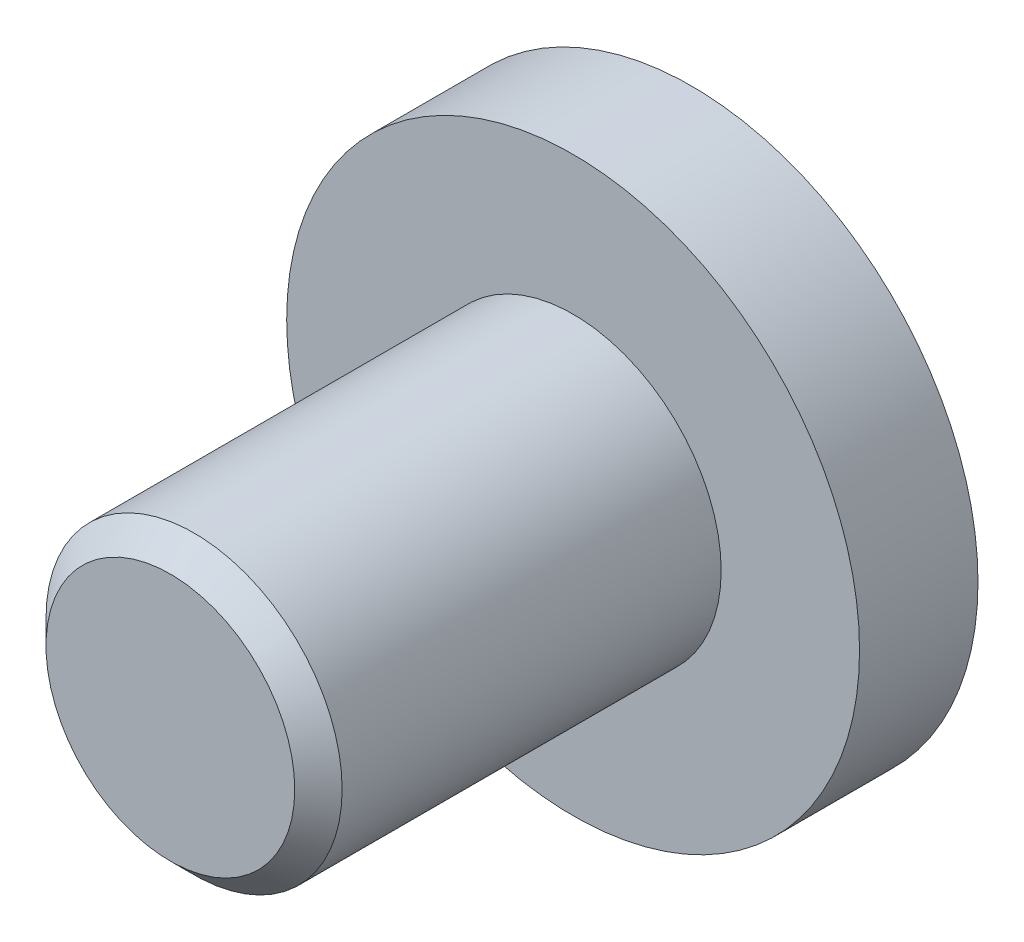
SolidWorks part; units mm, degrees
ref_plane "Front Plane" through (0, 0, 0) normal (0, 0, 1) x (1, 0, 0)
ref_plane "Top Plane" through (0, 0, 0) normal (0, 1, 0) x (1, 0, 0)
ref_plane "Right Plane" through (0, 0, 0) normal (1, 0, 0) x (0, 0, -1)
sketch "Sketch1" plane through (0, 0, 0) normal (0, 0, 1) x (1, 0, 0)
  circle A0 centre (0, 0) radius 12.0907
extrude "Boss-Extrude1" add sketch "Sketch1" along normal blind 5
sketch "Sketch2" plane through (0, 0, 5) normal (0, 0, 1) x (1, 0, 0)
  circle A0 centre (0, 0) radius 6.25
extrude "Boss-Extrude2" add sketch "Sketch2" along normal blind 17
chamfer "Chamfer1" distance 1 angle 45 1 edges at (6.25, 0, 22)
